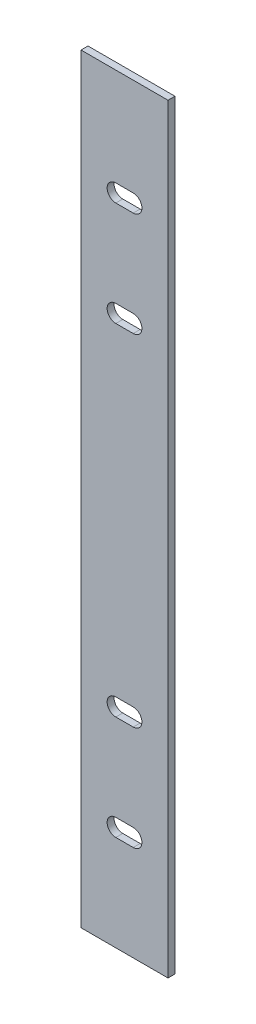
SolidWorks part; units mm, degrees
material "Q235B"
ref_plane "Front Plane" through (0, 0, 0) normal (0, 0, 1) x (1, 0, 0)
ref_plane "Top Plane" through (0, 0, 0) normal (0, 1, 0) x (1, 0, 0)
ref_plane "Right Plane" through (0, 0, 0) normal (1, 0, 0) x (0, 0, -1)
sketch "Sketch1" plane through (0, 0, 0) normal (0, 0, 1) x (1, 0, 0)
  line L0 (7408.9899, 2462.9859) -> (7408.9899, 4648.9859)
  line L1 (7658.9899, 2462.9859) -> (7658.9899, 4648.9859)
  line L2 (7508.9899, 4367.9859) -> (7558.9899, 4367.9859)
  line L3 (7508.9901, 4317.9859) -> (7558.9899, 4317.9859)
  line L4 (7508.9901, 3087.9859) -> (7558.9893, 3087.9859)
  line L5 (7558.9899, 3037.9859) -> (7508.9899, 3037.9859)
  line L6 (7508.9899, 4067.9859) -> (7558.9899, 4067.9859)
  line L7 (7508.9901, 4017.9859) -> (7558.9899, 4017.9859)
  line L8 (7508.9899, 2787.9859) -> (7558.9893, 2787.9859)
  line L9 (7508.9899, 2737.9859) -> (7558.9899, 2737.9859)
  line L10 (7408.9899, 4648.9859) -> (7658.9899, 4648.9859)
  line L11 (7408.9899, 2462.9859) -> (7658.9899, 2462.9859)
  arc A0 (7558.9899, 2737.9859) -> (7558.9893, 2787.9859) centre (7558.9896, 2762.9859) ccw
  arc A1 (7508.9899, 2787.9859) -> (7508.9899, 2737.9859) centre (7508.9898, 2762.9859) ccw
  arc A2 (7558.9899, 3037.9859) -> (7558.9893, 3087.9859) centre (7558.9896, 3062.9859) ccw
  arc A3 (7508.9901, 3087.9859) -> (7508.9899, 3037.9859) centre (7508.9899, 3062.9859) ccw
  arc A4 (7558.9899, 4017.9859) -> (7558.9899, 4067.9859) centre (7558.9899, 4042.9859) ccw
  arc A5 (7508.9899, 4067.9859) -> (7508.9901, 4017.9859) centre (7508.9896, 4042.9859) ccw
  arc A6 (7558.9899, 4317.9859) -> (7558.9899, 4367.9859) centre (7558.9899, 4342.9859) ccw
  arc A7 (7508.9899, 4367.9859) -> (7508.9901, 4317.9859) centre (7508.9896, 4342.9859) ccw
  dimension "D1" = 250
extrude "Boss-Extrude1" add sketch "Sketch1" along normal blind 20
